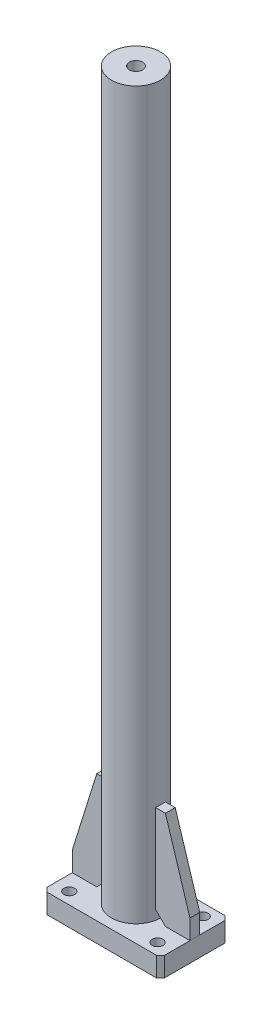
SolidWorks part; units mm, degrees
material "45#"
ref_plane "前基準面" through (0, 0, 0) normal (0, 0, 1) x (1, 0, 0)
ref_plane "上基準面" through (0, 0, 0) normal (0, 1, 0) x (1, 0, 0)
ref_plane "右基準面" through (0, 0, 0) normal (1, 0, 0) x (0, 0, -1)
sketch "草图1" plane through (0, 0, 0) normal (0, 1, 0) x (1, 0, 0)
  circle A0 centre (0, 0) radius 12.5
  dimension "D1" = 25
extrude "凸台-拉伸1" add sketch "草图1" along normal blind 370
sketch "草图2" plane through (0, 0, 0) normal (0, -1, 0) x (1, 0, 0)
  line L1 (30, -17.5) -> (-30, -17.5)
  line L2 (30, -17.5) -> (30, 17.5)
  line L3 (30, 17.5) -> (-30, 17.5)
  line L4 (-30, -17.5) -> (-30, 17.5)
  line L5 (30, -17.5) -> (-30, 17.5) construction
  line L6 (30, 17.5) -> (-30, -17.5) construction
  point P0 (0, 0)
  dimension "D1" = 35
  dimension "D2" = 60
extrude "凸台-拉伸2" add sketch "草图2" along normal blind 10 separate body
sketch "草图3" plane through (0, 0, 0) normal (0, 0, 1) x (1, 0, 0)
  line L0 (30, 0) -> (30, 10)
  line L1 (30, 10) -> (17.5, 50)
  line L2 (17.5, 50) -> (12.5, 50)
  line L3 (12.5, 0) -> (12.5, 370) construction
  line L4 (12.5, 50) -> (12.5, 5)
  line L5 (30, 0) -> (-30, 0) construction
  line L6 (17.5, 0) -> (30, 0)
  line L7 (12.5, 5) -> (17.5, 0)
  line L8 (0, 0) -> (0, 95.8558) construction
  line L9 (-12.5, 5) -> (-17.5, 0)
  line L10 (-17.5, 0) -> (-30, 0)
  line L11 (-12.5, 50) -> (-12.5, 5)
  line L12 (-17.5, 50) -> (-12.5, 50)
  line L13 (-30, 10) -> (-17.5, 50)
  line L14 (-30, 0) -> (-30, 10)
  point P8 (12.5, 0)
  point P15 (-12.5, 0)
  dimension "D1" = 10
  dimension "D2" = 5
  dimension "D3" = 50
extrude "凸台-拉伸3" add sketch "草图3" along normal mid plane 5 separate body
hole_wizard "M5 间隙孔1" positions "草图4" profile "草图5" hole size "M5" standard "GB" end condition up to next
sketch "草图4" plane through (0, -10, 0) normal (0, -1, 0) x (-1, 0, 0)
  line L1 (0, 0) -> (-42.4575, 0) construction
  line L3 (0, 0) -> (0, 29.4504) construction
  line L4 (-30, -17.5) -> (30, -17.5) construction
  line L5 (-30, 17.5) -> (-30, -17.5) construction
  point P24 (-22.5, -11.5)
  point P27 (-22.5, 11.5)
  point P28 (22.5, 11.5)
  point P29 (22.5, -11.5)
  dimension "D1" = 6
  dimension "D2" = 7.5
sketch "草图5" plane through (-22.5, -10, 11.5) normal (1, 0, 0) x (0, 0, -1)
  line L0 (0, 0) -> (0, 10.001)
  line L1 (0, 10.001) -> (2.75, 10.001)
  line L2 (2.75, 10.001) -> (2.75, 0)
  line L5 (2.75, 0) -> (0, 0)
  line L11 (0, -6.35) -> (0, 107.95) construction
  dimension "通孔孔直径" = 5.5
  dimension "通孔孔深度" = 10.001
hole_wizard "M8 螺纹孔1" positions "草图6" profile "草图7" tap size "M8" standard "GB"
sketch "草图6" plane through (0, 370, 0) normal (0, 1, 0) x (1, 0, 0)
  point P0 (0, 0)
cosmetic thread "孔螺蚊线1" parameters "D1"=16, "D2"=8
sketch "草图7" plane through (0, 370, 0) normal (1, 0, 0) x (0, 0, 1)
  line L0 (0, 0) -> (0, 21.7929)
  line L1 (0, 21.7929) -> (3.4, 19.75)
  line L2 (3.4, 19.75) -> (3.4, 0)
  line L5 (3.4, 0) -> (0, 0)
  line L10 (0, 21.7929) -> (-3.4, 19.75) construction
  line L11 (0, -6.35) -> (0, 107.95) construction
  dimension "螺纹孔钻头直径" = 6.8
  dimension "螺纹孔钻头深度" = 19.75
  dimension "导头角度" = 118
chamfer "倒角1" distance 2 angle 45 4 edges at (-30, -5, -17.5) (-30, -5, 17.5) (30, -5, -17.5) (30, -5, 17.5)
